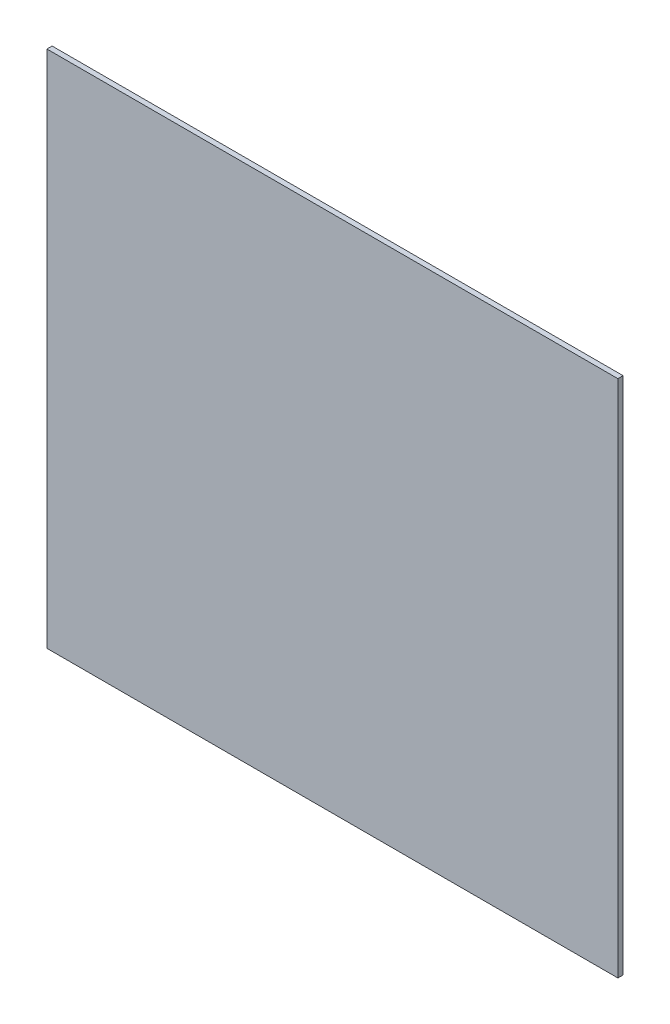
from build123d import *

# Parameters (mm, degrees)
SKETCH1_W           = 220
SKETCH1_H           = 200
BOSS_EXTRUDE1_DEPTH = 2


with BuildPart() as part:
    # Sketch1 → Boss-Extrude1 (new body)
    with BuildSketch(Plane.XY):
        with Locations((-13.680151025, 9)):
            Rectangle(SKETCH1_W, SKETCH1_H)
    extrude(amount=BOSS_EXTRUDE1_DEPTH)


solid = part.part
